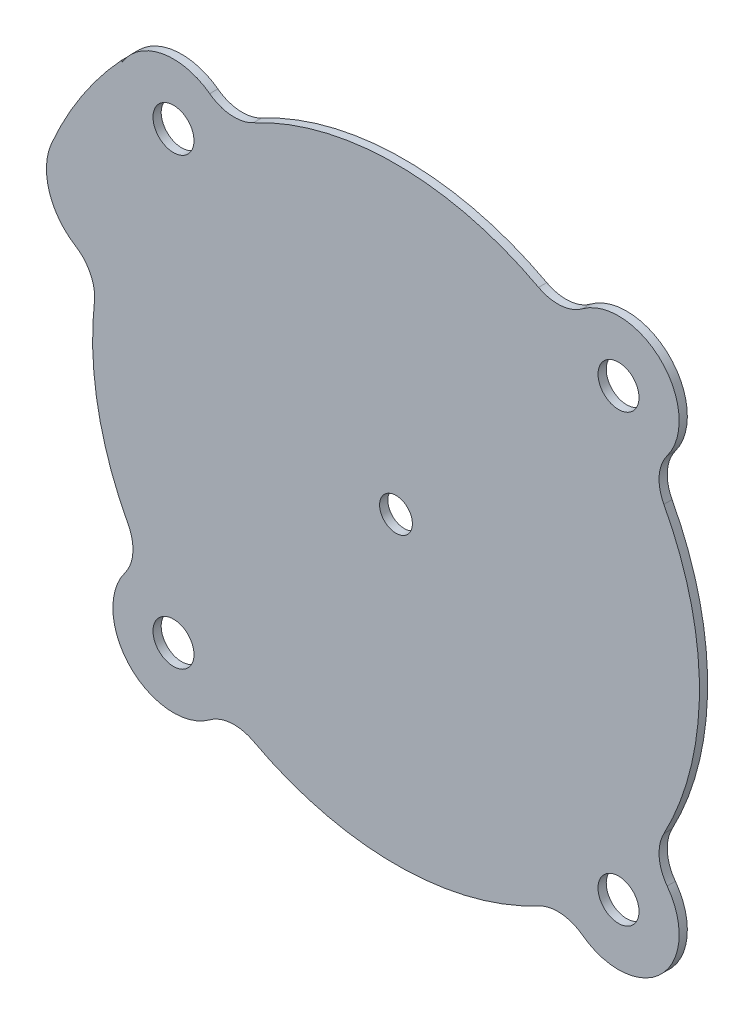
SolidWorks part; units mm, degrees
material "BUTYL"
ref_plane "Front Plane" through (0, 0, 0) normal (0, 0, 1) x (1, 0, 0)
ref_plane "Top Plane" through (0, 0, 0) normal (0, 1, 0) x (1, 0, 0)
ref_plane "Right Plane" through (0, 0, 0) normal (1, 0, 0) x (0, 0, -1)
sketch "Sketch1" plane through (0, 0, 0) normal (0, 0, 1) x (1, 0, 0)
  line L2 (-33.3881, 31.0734) -> (-33.4549, 31.2278)
  arc A5 (-29.6334, -27.1334) -> (-28.9012, -28.9012) centre (-27.1334, -27.1334) ccw
  arc A6 (27.1334, -29.6334) -> (28.9012, -28.9012) centre (27.1334, -27.1334) ccw
  arc A7 (-27.1334, 29.6334) -> (-28.9012, 28.9012) centre (-27.1334, 27.1334) ccw
  arc A10 (28.9012, 28.9012) -> (29.6334, 27.1334) centre (27.1334, 27.1334) ccw
  arc A11 (29.6334, 27.1334) -> (28.9012, 28.9012) centre (27.1334, 27.1334) ccw
  arc A36 (-42.0118, 18.1497) -> (-39.1008, 8.8147) centre (-35.1268, 15.1753) ccw
  arc A37 (-36.7799, 4.0298) -> (-39.1008, 8.8147) centre (-41.7502, 4.5743) ccw
  arc A38 (-36.7799, 4.0298) -> (-32.661, -17.3855) centre (0, 0) ccw
  arc A39 (-33.0636, -22.7201) -> (-32.661, -17.3855) centre (-37.0747, -19.7349) ccw
  arc A40 (-33.0636, -22.7201) -> (-22.7201, -33.0636) centre (-27.1334, -27.1334) ccw
  arc A41 (-17.3855, -32.661) -> (-22.7201, -33.0636) centre (-19.7349, -37.0747) ccw
  arc A42 (-17.3855, -32.661) -> (17.3855, -32.661) centre (0, 0) ccw
  arc A43 (22.7201, -33.0636) -> (17.3855, -32.661) centre (19.7349, -37.0747) ccw
  arc A44 (22.7201, -33.0636) -> (33.0636, -22.7201) centre (27.1334, -27.1334) ccw
  arc A45 (32.661, -17.3855) -> (33.0636, -22.7201) centre (37.0747, -19.7349) ccw
  arc A46 (32.661, -17.3855) -> (32.661, 17.3855) centre (0, 0) ccw
  arc A47 (33.0636, 22.7201) -> (32.661, 17.3855) centre (37.0747, 19.7349) ccw
  arc A48 (33.0636, 22.7201) -> (22.7201, 33.0636) centre (27.1334, 27.1334) ccw
  arc A49 (17.3855, 32.661) -> (22.7201, 33.0636) centre (19.7349, 37.0747) ccw
  arc A50 (17.3855, 32.661) -> (-17.3855, 32.661) centre (0, 0) ccw
  arc A51 (-22.7201, 33.0636) -> (-17.3855, 32.661) centre (-19.7349, 37.0747) ccw
  arc A52 (-22.7201, 33.0636) -> (-33.3881, 31.0734) centre (-27.1334, 27.1334) ccw
  arc A53 (-33.4549, 31.2278) -> (-42.0118, 18.1497) centre (0, 0) ccw
  spline S3 degree 2 poles (-28.9012, -28.9012) (-28.169, -29.6334) (-27.1334, -29.6334) (-26.0979, -29.6334) (-25.3657, -28.9012) (-24.6334, -28.169) (-24.6334, -27.1334) (-24.6334, -26.0979) (-25.3657, -25.3657) (-26.0979, -24.6334) (-27.1334, -24.6334) (-28.169, -24.6334) (-28.9012, -25.3657) (-29.6334, -26.0979) (-29.6334, -27.1334) knots 0.941667 0.941667 0.941667 0.95 0.95 0.958333 0.958333 0.966667 0.966667 0.975 0.975 0.983333 0.983333 0.991667 0.991667 1 1 1 weights 1 0.92388 1 0.92388 1 0.92388 1 0.92388 1 0.92388 1 0.92388 1 0.92388 1
  spline S4 degree 2 poles (28.9012, -28.9012) (29.6334, -28.169) (29.6334, -27.1334) (29.6334, -26.0979) (28.9012, -25.3657) (28.169, -24.6334) (27.1334, -24.6334) (26.0979, -24.6334) (25.3657, -25.3657) (24.6334, -26.0979) (24.6334, -27.1334) (24.6334, -28.169) (25.3657, -28.9012) (26.0979, -29.6334) (27.1334, -29.6334) knots 0.941667 0.941667 0.941667 0.95 0.95 0.958333 0.958333 0.966667 0.966667 0.975 0.975 0.983333 0.983333 0.991667 0.991667 1 1 1 weights 1 0.92388 1 0.92388 1 0.92388 1 0.92388 1 0.92388 1 0.92388 1 0.92388 1
  spline S5 degree 2 poles (-28.9012, 28.9012) (-29.6334, 28.169) (-29.6334, 27.1334) (-29.6334, 26.0979) (-28.9012, 25.3657) (-28.169, 24.6334) (-27.1334, 24.6334) (-26.0979, 24.6334) (-25.3657, 25.3657) (-24.6334, 26.0979) (-24.6334, 27.1334) (-24.6334, 28.169) (-25.3657, 28.9012) (-26.0979, 29.6334) (-27.1334, 29.6334) knots 0.941667 0.941667 0.941667 0.95 0.95 0.958333 0.958333 0.966667 0.966667 0.975 0.975 0.983333 0.983333 0.991667 0.991667 1 1 1 weights 1 0.92388 1 0.92388 1 0.92388 1 0.92388 1 0.92388 1 0.92388 1 0.92388 1
extrude "Boss-Extrude1" add sketch "Sketch1" along normal blind 1
sketch "Sketch2" plane through (0, 0, 0) normal (0, 0, -1) x (-1, 0, 0)
  circle A0 centre (0, 0) radius 2
extrude "Cut-Extrude1" cut sketch "Sketch2" against normal blind 1
